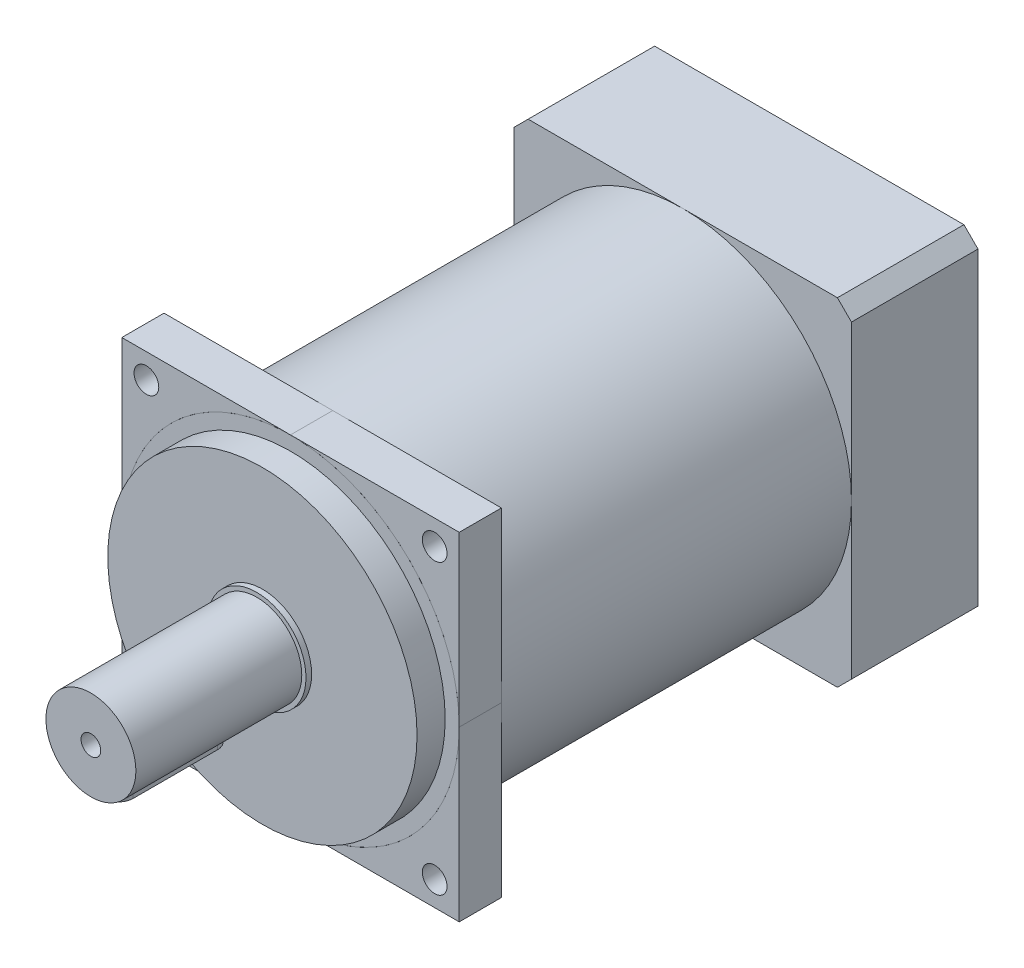
from build123d import *

# Parameters (mm, degrees)
SKETCH1_W                 = 120
SKETCH1_H                 = 120
EXTRUDE1_DEPTH            = 45
SKETCH2_R                 = 60
EXTRUDE2_DEPTH            = 139.5
SKETCH3_R                 = 55
EXTRUDE3_DEPTH            = 10
SKETCH4_R                 = 17.5
EXTRUDE4_DEPTH            = 2
SKETCH5_R                 = 16
EXTRUDE5_DEPTH            = 59
CHAMFER1_SIZE             = 5
M8X1_0_TAPPED_HOLE1_D     = 7
M8X1_0_TAPPED_HOLE1_DEPTH = 19
M8X1_0_TAPPED_HOLE1_TIP   = 2.103012167
EXTRUDE6_DEPTH            = 3
SKETCH19_R                = 5
CUT_EXTRUDE1_DEPTH        = 10
SKETCH20_R                = 55
CUT_EXTRUDE2_DEPTH        = 7
CIRPATTERN1_COUNT         = 4
BOSS_EXTRUDE1_DEPTH       = 15
BOSS_EXTRUDE1_2_DEPTH     = 15
BOSS_EXTRUDE1_3_DEPTH     = 15
BOSS_EXTRUDE1_4_DEPTH     = 15
SKETCH24_R                = 4.4
CUT_EXTRUDE3_DEPTH        = 15
CIRPATTERN2_COUNT         = 4


with BuildPart() as part:
    # Sketch1 → Extrude1 (new body)
    with BuildSketch(Plane.XY):
        with Locations((60, -60)):
            Rectangle(SKETCH1_W, SKETCH1_H)
    extrude(amount=EXTRUDE1_DEPTH)

    # Sketch2 → Extrude2 (add)
    with BuildSketch(Plane.XY.offset(45)):
        with Locations((60, -60)):
            Circle(SKETCH2_R)
    extrude(amount=EXTRUDE2_DEPTH)

    # Sketch3 → Extrude3 (add)
    with BuildSketch(Plane.XY.offset(184.5)):
        with Locations((60, -60)):
            Circle(SKETCH3_R)
    extrude(amount=EXTRUDE3_DEPTH)

    # Sketch4 → Extrude4 (add)
    with BuildSketch(Plane.XY.offset(194.5)):
        with Locations((60, -60)):
            Circle(SKETCH4_R)
    extrude(amount=EXTRUDE4_DEPTH)

    # Sketch5 → Extrude5 (add)
    with BuildSketch(Plane.XY.offset(196.5)):
        with Locations((60, -60)):
            Circle(SKETCH5_R)
    extrude(amount=EXTRUDE5_DEPTH)

    # Chamfer1
    chamfer1_edges = [part.edges().sort_by_distance(p)[0] for p in [
        (0, 0, 22.5),
        (120, 0, 22.5),
        (120, -120, 22.5),
        (0, -120, 22.5),
    ]]
    chamfer(chamfer1_edges, length=CHAMFER1_SIZE)

    # M8x1.0 Tapped Hole1
    with Locations(Plane.XY.offset(255.5)):
        with Locations((60, -60)):
            Hole(M8X1_0_TAPPED_HOLE1_D / 2, depth=M8X1_0_TAPPED_HOLE1_DEPTH)
            with Locations((0, 0, -(M8X1_0_TAPPED_HOLE1_DEPTH + M8X1_0_TAPPED_HOLE1_TIP / 2))):  # 118° drill point
                Cone(0, M8X1_0_TAPPED_HOLE1_D / 2, M8X1_0_TAPPED_HOLE1_TIP, mode=Mode.SUBTRACT)

    # Sketch19 → Cut-Extrude1 (cut)
    with BuildSketch(Plane.ZY):
        with Locations(Location((10, -20, 0), (0, 0, 270))):
            Circle(SKETCH19_R)
    extrude(amount=-CUT_EXTRUDE1_DEPTH, mode=Mode.SUBTRACT)

    # Sketch20 → Cut-Extrude2 (cut)
    with BuildSketch(Plane(origin=(0, 0, 0), x_dir=(-1, 0, 0), z_dir=(0, 0, -1))):
        with Locations(Location((-60, -60, 0), (0, 0, 180))):
            Circle(SKETCH20_R)
    extrude(amount=-CUT_EXTRUDE2_DEPTH, mode=Mode.SUBTRACT)

    # Sketch21 → M8 Tapped Hole1 (revolve, cut)
    with BuildSketch(Plane(origin=(111.265241636, -8.734758364, 0), x_dir=(0, 1, 0), z_dir=(1, 0, 0))):
        Polygon((0, 0), (0, 21.792926105), (3.4, 19.75), (3.4, 0), align=None)
    m8_tapped_hole1 = revolve(axis=Axis((111.265241636, -8.734758364, -6.35), (0, 0, 1)), mode=Mode.SUBTRACT)

    # CirPattern1: M8 Tapped Hole1 ×4 about axis
    cirpattern1_axis = Axis((60, -60, 0), (0, 0, 1))
    for i in range(1, CIRPATTERN1_COUNT):
        add(m8_tapped_hole1.rotate(cirpattern1_axis, i * 360 / CIRPATTERN1_COUNT), mode=Mode.SUBTRACT)


with BuildPart() as body_2:
    # Sketch18 → Extrude6 (new body)
    with BuildSketch(Plane.XZ.offset(76)):
        with BuildLine():
            Line((55, 245.5), (55, 215.5))
            ThreePointArc((55, 215.5), (60, 210.5), (65, 215.5))
            Line((65, 215.5), (65, 245.5))
            ThreePointArc((65, 245.5), (60, 250.5), (55, 245.5))
        make_face()
    extrude(amount=EXTRUDE6_DEPTH)


with BuildPart() as body_3:
    # Sketch23 → Boss-Extrude1 (new body)
    with BuildSketch(Plane.XY.offset(184.5)):
        with BuildLine():
            Line((120, 0), (60, 0))
            ThreePointArc((60, 0), (102.426406871, -17.573593129), (120, -60))
            Line((120, -60), (120, 0))
        make_face()
    extrude(amount=-BOSS_EXTRUDE1_DEPTH)


with BuildPart() as body_4:
    # Sketch23 → Boss-Extrude1 2 (new body)
    with BuildSketch(Plane.XY.offset(184.5)):
        with BuildLine():
            Line((60, 0), (0, 0))
            Line((0, 0), (0, -60.000000158))
            ThreePointArc((0, -60.000000158), (17.573593073, -17.573593185), (60, 0))
        make_face()
    extrude(amount=-BOSS_EXTRUDE1_2_DEPTH)

    # Sketch24 → Cut-Extrude3 (cut)
    with BuildSketch(Plane.XY.offset(184.5)):
        with Locations((8.734758364, -8.734758364)):
            Circle(SKETCH24_R)
    cut_extrude3 = extrude(amount=-CUT_EXTRUDE3_DEPTH, mode=Mode.SUBTRACT)


with BuildPart() as body_5:
    # Sketch23 → Boss-Extrude1 3 (new body)
    with BuildSketch(Plane.XY.offset(184.5)):
        with BuildLine():
            ThreePointArc((60, -120), (17.573593185, -102.426406927), (0, -60.000000158))
            Line((0, -60.000000158), (0, -120))
            Line((0, -120), (60, -120))
        make_face()
    extrude(amount=-BOSS_EXTRUDE1_3_DEPTH)


with BuildPart() as body_6:
    # Sketch23 → Boss-Extrude1 4 (new body)
    with BuildSketch(Plane.XY.offset(184.5)):
        with BuildLine():
            Line((120, -120), (120, -60))
            ThreePointArc((120, -60), (102.426406871, -102.426406871), (60, -120))
            Line((60, -120), (120, -120))
        make_face()
    extrude(amount=-BOSS_EXTRUDE1_4_DEPTH)


with BuildPart() as cirpattern2_tool:
    # CirPattern2: Cut-Extrude3 ×4 about axis
    cirpattern2_axis = Axis((60, -60, 0), (0, 0, 1))
    for i in range(1, CIRPATTERN2_COUNT):
        add(cut_extrude3.rotate(cirpattern2_axis, i * 360 / CIRPATTERN2_COUNT))


with BuildPart() as body_3_1:
    add(body_3.part)

    # CirPattern2: cut by cirpattern2_tool
    add(cirpattern2_tool.part, mode=Mode.SUBTRACT)


with BuildPart() as body_5_1:
    add(body_5.part)

    # CirPattern2: cut by cirpattern2_tool
    add(cirpattern2_tool.part, mode=Mode.SUBTRACT)


with BuildPart() as body_6_1:
    add(body_6.part)

    # CirPattern2: cut by cirpattern2_tool
    add(cirpattern2_tool.part, mode=Mode.SUBTRACT)


solid = Compound([part.part, body_2.part, body_4.part, body_3_1.part, body_5_1.part, body_6_1.part])
